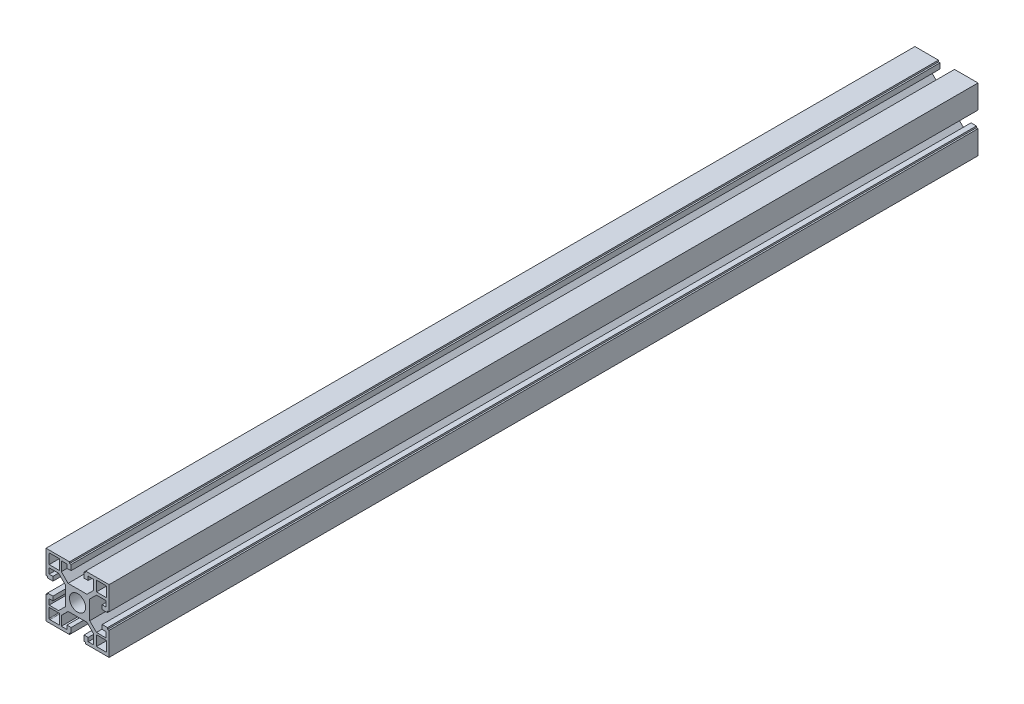
from build123d import *

# Parameters (mm, degrees)
SKETCH_1_W                  = 40
SKETCH_1_H                  = 40
EXTRUDE_1_DEPTH             = 551
HOLE_WIZARD_6_5_6_5_1_D     = 6.5
CUT_EXTRUDE_1_DEPTH         = 552.725475214
PATTERN_CIRCULAR_1_COUNT    = 4
SKETCH_5_W                  = 6.5
SKETCH_5_H                  = 6.5
CUT_EXTRUDE_2_DEPTH         = 552.725475214
PATTERN_LINEAR_1_COUNT      = 2
PATTERN_LINEAR_1_PITCH      = 30
PATTERN_LINEAR_1_COUNT_DIR2 = 2
PATTERN_LINEAR_1_PITCH_DIR2 = 30
FILLET_2_R                  = 0.5
HOLE_WIZARD_M12_1_D         = 10.2
HOLE_WIZARD_M12_1_DEPTH     = 29.25
HOLE_WIZARD_M12_1_TIP       = 3.064389157
HOLE_WIZARD_M8_2_D          = 6.8
HOLE_WIZARD_M8_2_DEPTH      = 19.75
HOLE_WIZARD_M8_2_TIP        = 2.042926105


with BuildPart() as part:
    # 草图1 → 凸台-拉伸1 (new body)
    with BuildSketch(Plane.XY):
        Rectangle(SKETCH_1_W, SKETCH_1_H)
    extrude(amount=EXTRUDE_1_DEPTH)

    # Ø6.5 (6.5) 直径孔1 (through all)
    with Locations(Plane.XY.offset(551)):
        with Locations((0, 0)):
            Hole(HOLE_WIZARD_6_5_6_5_1_D / 2)

    # 草图4 → 切除-拉伸1 (cut, through all)
    with BuildSketch(Plane.XY.offset(551)):
        Polygon((6, -7.7), (10.25, -12), (10.25, -18), (6.75, -18), (6.75, -15.6), (4.1, -15.6), (4.1, -19), (5.1, -19), (5.1, -23.725727051), (-5.1, -23.725727051), (-5.1, -19), (-4.1, -19), (-4.1, -15.6), (-6.75, -15.6), (-6.75, -18), (-10.25, -18), (-10.25, -12), (-6, -7.7), align=None)
    cut_extrude_1 = extrude(amount=-CUT_EXTRUDE_1_DEPTH, mode=Mode.SUBTRACT)

    # 阵列(圆周)1: 切除-拉伸1 ×4 about axis
    pattern_circular_1_axis = Axis((0, 0, 0), (0, 0, 1))
    for i in range(1, PATTERN_CIRCULAR_1_COUNT):
        add(cut_extrude_1.rotate(pattern_circular_1_axis, i * 360 / PATTERN_CIRCULAR_1_COUNT), mode=Mode.SUBTRACT)

    # 草图5 → 切除-拉伸2 (cut, through all)
    with BuildSketch(Plane(origin=(0, 0, 0), x_dir=(-1, 0, 0), z_dir=(0, 0, -1))):
        with Locations((14.75, -14.75)):
            Rectangle(SKETCH_5_W, SKETCH_5_H)
    cut_extrude_2 = extrude(amount=-CUT_EXTRUDE_2_DEPTH, mode=Mode.SUBTRACT)

    # 阵列(线性)1: Cut-Extrude 2 2 × 2
    with Locations(*[(i * PATTERN_LINEAR_1_PITCH, j * PATTERN_LINEAR_1_PITCH_DIR2, 0) for i in range(PATTERN_LINEAR_1_COUNT) for j in range(PATTERN_LINEAR_1_COUNT_DIR2) if (i, j) != (0, 0)]):
        add(cut_extrude_2, mode=Mode.SUBTRACT)

    # 圆角2
    fillet_2_edges = [part.edges().sort_by_distance(p)[0] for p in [
        (-18, -18, 275.5),
        (18.5, -18, 275.5),
        (-18, 18.5, 275.5),
        (18.5, 18.5, 275.5),
    ]]
    fillet(fillet_2_edges, radius=FILLET_2_R)

    # M12 螺纹孔1
    with Locations(Plane.XY.offset(551)):
        with Locations((0, 0)):
            Hole(HOLE_WIZARD_M12_1_D / 2, depth=HOLE_WIZARD_M12_1_DEPTH)
            with Locations((0, 0, -(HOLE_WIZARD_M12_1_DEPTH + HOLE_WIZARD_M12_1_TIP / 2))):  # 118° drill point
                Cone(0, HOLE_WIZARD_M12_1_D / 2, HOLE_WIZARD_M12_1_TIP, mode=Mode.SUBTRACT)

    # M8 螺纹孔2
    with Locations(Plane(origin=(0, 0, 0), x_dir=(-1, 0, 0), z_dir=(0, 0, -1))):
        with Locations((0, 0)):
            Hole(HOLE_WIZARD_M8_2_D / 2, depth=HOLE_WIZARD_M8_2_DEPTH)
            with Locations((0, 0, -(HOLE_WIZARD_M8_2_DEPTH + HOLE_WIZARD_M8_2_TIP / 2))):  # 118° drill point
                Cone(0, HOLE_WIZARD_M8_2_D / 2, HOLE_WIZARD_M8_2_TIP, mode=Mode.SUBTRACT)


solid = part.part
